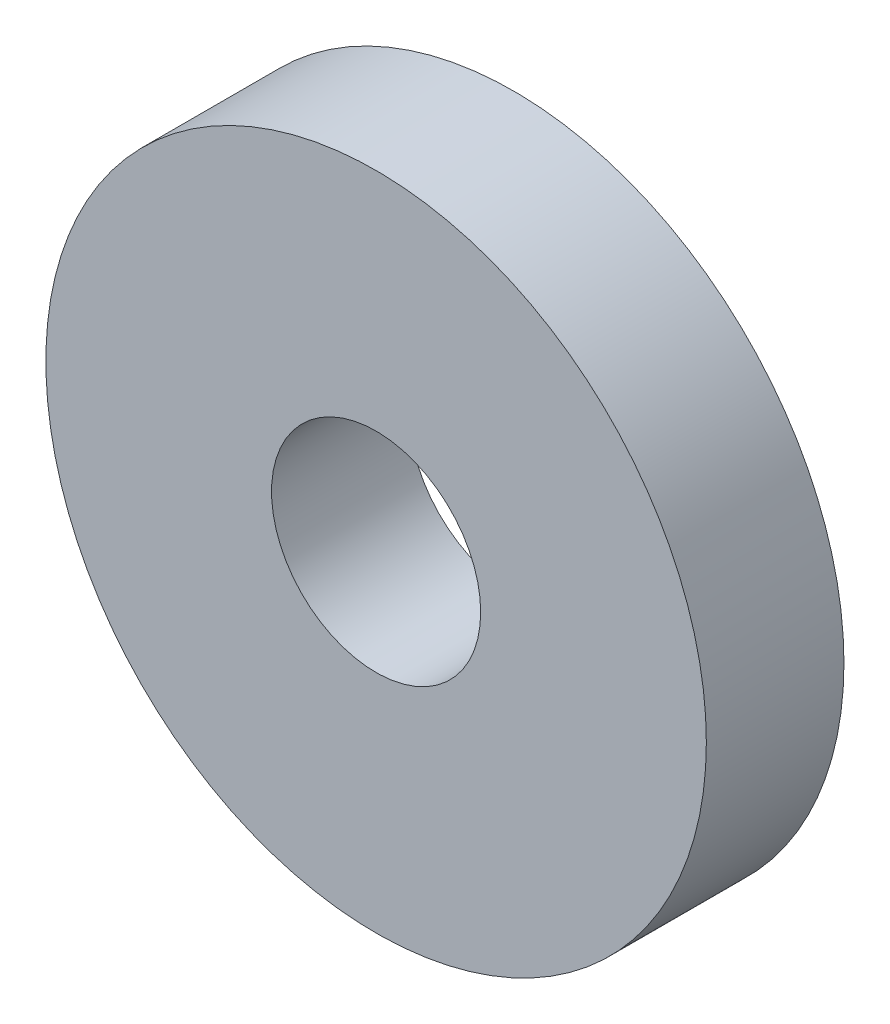
SolidWorks part; units mm, degrees
ref_plane "前视基准面" through (0, 0, 0) normal (0, 0, 1) x (1, 0, 0)
ref_plane "上视基准面" through (0, 0, 0) normal (0, 1, 0) x (1, 0, 0)
ref_plane "右视基准面" through (0, 0, 0) normal (1, 0, 0) x (0, 0, -1)
sketch "草图1" plane through (0, 0, 0) normal (0, 0, 1) x (1, 0, 0)
  arc A0 (-23.9728, -1.1429) -> (23.9728, -1.1429) centre (0, 0) ccw
  circle A1 centre (0, 0) radius 7.6
  arc A2 (23.9728, -1.1429) -> (-23.9728, -1.1429) centre (0, 0) ccw
  point P7 (0, 0)
  dimension "D1" = 48
  dimension "D2" = 15.2
extrude "凸台-拉伸1" add sketch "草图1" along normal blind 10
